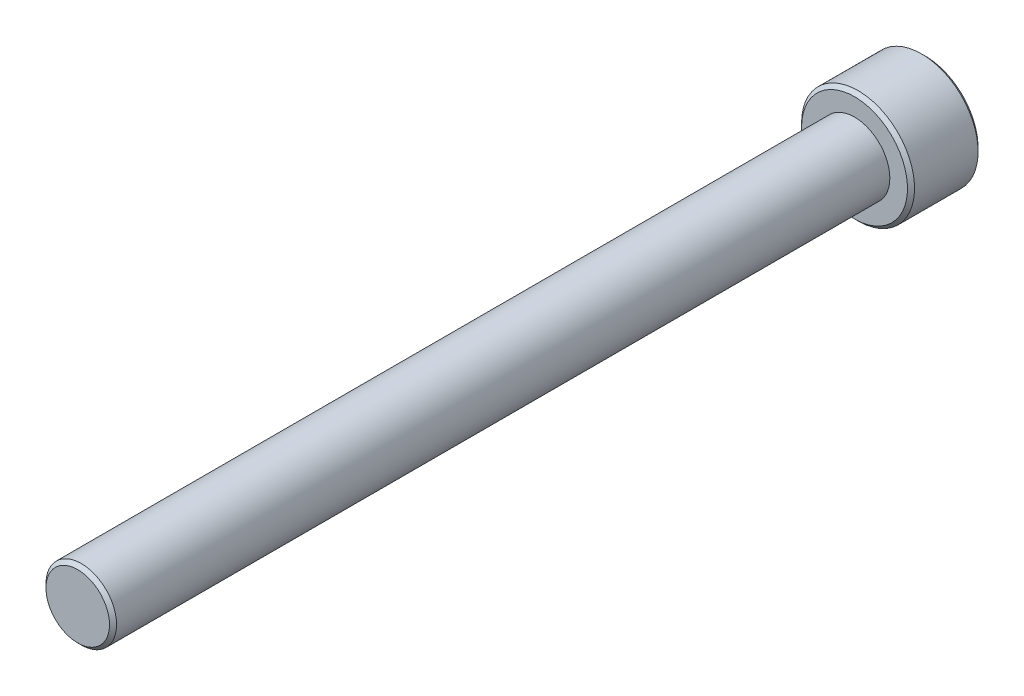
from build123d import *

# Parameters (mm, degrees)
SKETCH1_R           = 5
BOSS_EXTRUDE1_DEPTH = 110
SKETCH2_R           = 8
BOSS_EXTRUDE2_DEPTH = 10
CHAMFER1_SIZE       = 0.5


with BuildPart() as part:
    # Sketch1 → Boss-Extrude1 (new body)
    with BuildSketch(Plane.XY):
        Circle(SKETCH1_R)
    extrude(amount=BOSS_EXTRUDE1_DEPTH)

    # Sketch2 → Boss-Extrude2 (add)
    with BuildSketch(Plane(origin=(0, 0, 0), x_dir=(-1, 0, 0), z_dir=(0, 0, -1))):
        Circle(SKETCH2_R)
    extrude(amount=BOSS_EXTRUDE2_DEPTH)

    # Chamfer1
    chamfer1_edges = [part.edges().sort_by_distance(p)[0] for p in [
        (-5, 0, 110),
        (8, 0, 0),
        (8, 0, -10),
    ]]
    chamfer(chamfer1_edges, length=CHAMFER1_SIZE)


solid = part.part
